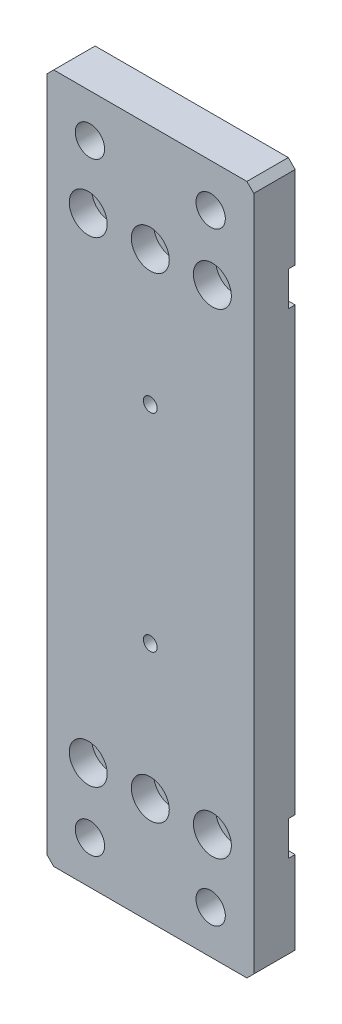
SolidWorks part; units mm, degrees
ref_plane "Front Plane" through (0, 0, 0) normal (0, 0, 1) x (1, 0, 0)
ref_plane "Top Plane" through (0, 0, 0) normal (0, 1, 0) x (1, 0, 0)
ref_plane "Right Plane" through (0, 0, 0) normal (1, 0, 0) x (0, 0, -1)
sketch "Sketch1" plane through (0, 0, 0) normal (0, 0, 1) x (1, 0, 0)
  line L1 (-30, -100) -> (30, -100)
  line L2 (-30, -100) -> (-30, 100)
  line L3 (-30, 100) -> (30, 100)
  line L4 (30, -100) -> (30, 100)
  line L5 (-30, -100) -> (30, 100) construction
  line L6 (-30, 100) -> (30, -100) construction
  point P0 (0, 0)
  dimension "D1" = 200
  dimension "D2" = 60
extrude "Boss-Extrude1" add sketch "Sketch1" along normal mid plane 12
chamfer "Chamfer1" distance 2 angle 45 4 edges at (30, 100, 0) (-30, 100, 0) (30, -100, 0) (-30, -100, 0)
sketch "Sketch2" plane through (0, 0, -6) normal (0, 0, -1) x (-1, 0, 0)
  line L0 (30, 98) -> (30, -98) construction
  line L1 (30, 74) -> (-30, 74)
  line L2 (30, 74) -> (30, 64)
  line L3 (30, 64) -> (-30, 64)
  line L4 (-30, 74) -> (-30, 64)
  line L5 (-30, -98) -> (-30, 98) construction
  line L6 (0, 0) -> (56.4067, 0) construction
  line L7 (-30, -64) -> (30, -64)
  line L8 (-30, -64) -> (-30, -74)
  line L9 (-30, -74) -> (30, -74)
  line L10 (30, -64) -> (30, -74)
  dimension "D1" = 10
  dimension "D2" = 138
extrude "Cut-Extrude1" cut sketch "Sketch2" against normal blind 2
hole_wizard "Hole size per socket head cap screw type 1" positions "Sketch4" profile "Sketch3" counterbore size "M6" standard "Gb" end condition through all
sketch "Sketch4" plane through (0, 0, 6) normal (0, 0, 1) x (1, 0, 0)
  point P0 (-18, -69)
  point P3 (0, -69)
  point P6 (18, -69)
  point P9 (18, 69)
  point P12 (0, 69)
  point P15 (-18, 69)
sketch "Sketch3" plane through (-18, -69, 6) normal (1, 0, 0) x (0, -1, 0)
  line L0 (0, 0) -> (0, 12)
  line L1 (0, 12) -> (3.25, 12)
  line L3 (3.25, 12) -> (3.25, 6.5)
  line L4 (3.25, 6.5) -> (5.5, 6.5)
  line L5 (5.5, 6.5) -> (5.5, 0)
  line L7 (5.5, 0) -> (0, 0)
  line L11 (0, -6.35) -> (0, 107.95) construction
  dimension "通孔孔直径" = 6.5
  dimension "通孔孔深度" = 12
  dimension "柱形沉头孔直径" = 11
  dimension "柱形沉头孔深度" = 6.5
sketch "Sketch5" plane through (0, 0, -6) normal (0, 0, -1) x (-1, 0, 0)
  line L1 (17.5, 87.5) -> (-17.5, 87.5) construction
  line L2 (17.5, 87.5) -> (17.5, -87.5) construction
  line L3 (17.5, -87.5) -> (-17.5, -87.5) construction
  line L4 (-17.5, 87.5) -> (-17.5, -87.5) construction
  line L5 (17.5, 87.5) -> (-17.5, -87.5) construction
  line L6 (17.5, -87.5) -> (-17.5, 87.5) construction
  circle A0 centre (17.5, 87.5) radius 4.25
  circle A1 centre (-17.5, 87.5) radius 4.25
  circle A2 centre (17.5, -87.5) radius 4.25
  circle A3 centre (-17.5, -87.5) radius 4.25
  point P0 (0, 0)
  dimension "D3" = 8.5
  dimension "D1" = 175
  dimension "D2" = 35
extrude "Cut-Extrude2" cut sketch "Sketch5" against normal through all
sketch "Sketch6" plane through (0, 0, 6) normal (0, 0, 1) x (1, 0, 0)
  circle A0 centre (0, 30) radius 2
  circle A1 centre (0, -30) radius 2
  dimension "D1" = 4
  dimension "D2" = 60
  dimension "D3" = 30
extrude "Cut-Extrude3" cut sketch "Sketch6" against normal through all
